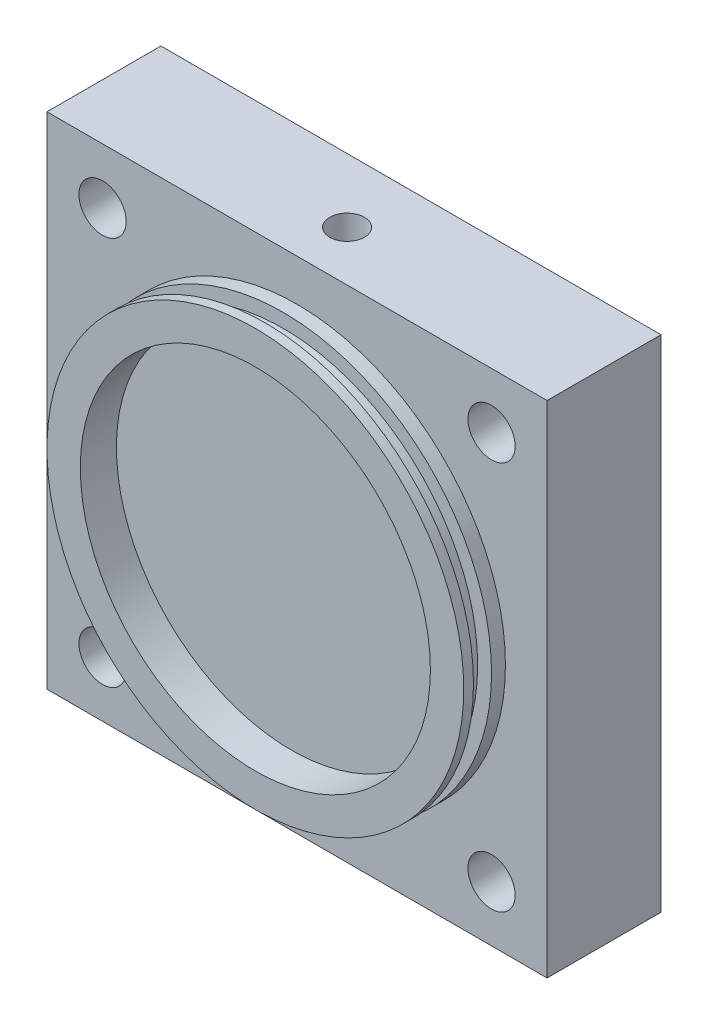
from build123d import *

# Parameters (mm, degrees)
SKETCH_1_W               = 180
SKETCH_1_H               = 180
EXTRUDE_1_DEPTH          = 41
SKETCH_2_R               = 75
EXTRUDE_2_DEPTH          = 15
SKETCH_3_R               = 63
CUT_EXTRUDE_1_DEPTH      = 13
SKETCH_4_W               = 6.5
SKETCH_4_H               = 5
CUT_EXTRUDE_2_REACH      = 136.347
CUT_EXTRUDE_2_END_RADIUS = 5.5626
SKETCH_9_R               = 3
CUT_EXTRUDE_4_REACH      = 141.054
SKETCH_11_R              = 8.5


with BuildPart() as part:
    # 草图1 → 凸台-拉伸1 (new body)
    with BuildSketch(Plane.XY):
        Rectangle(SKETCH_1_W, SKETCH_1_H)
    extrude(amount=EXTRUDE_1_DEPTH)

    # 草图2 → 凸台-拉伸2 (add)
    with BuildSketch(Plane.XY.offset(41)):
        Circle(SKETCH_2_R)
    extrude(amount=EXTRUDE_2_DEPTH)

    # 草图3 → 切除-拉伸1 (cut)
    with BuildSketch(Plane.XY.offset(56)):
        Circle(SKETCH_3_R)
    extrude(amount=-CUT_EXTRUDE_1_DEPTH, mode=Mode.SUBTRACT)

    # 草图4 → 切除-旋转1 (revolve, cut)
    with BuildSketch(Plane(origin=(0, 0, 0), x_dir=(0, 0, -1), z_dir=(1, 0, 0)), mode=Mode.PRIVATE) as cut_revolve_1_sk:
        with Locations((-49.25, 72.5)):
            Rectangle(SKETCH_4_W, SKETCH_4_H)
    revolve(cut_revolve_1_sk.sketch.rotate(Axis((0, 0, 56), (0, 0, -1)), 90), axis=Axis((0, 0, 56), (0, 0, -1)), mode=Mode.SUBTRACT)

    # 草图6 → 1/4 NPT 螺纹孔1 (revolve, cut)
    with BuildSketch(Plane(origin=(0, 90, 23), x_dir=(0, 0, 1), z_dir=(1, 0, 0))):
        Polygon((0, 0), (0, 36.342347279), (5.5626, 33), (5.5626, 10.02), (5.943676082, 10.02), (6.2436883, 0), align=None)
    revolve(axis=Axis((0, 96.35, 23), (0, -1, 0)), mode=Mode.SUBTRACT)

    # 切除-拉伸2: up to this cylinder (the profile starts outside it)
    cut_extrude_2_end = Plane(origin=(0, 60, 23), z_dir=(0, 1, 0)) * Cylinder(CUT_EXTRUDE_2_END_RADIUS, 284.8192, mode=Mode.PRIVATE)
    # 草图9 → 切除-拉伸2 (cut, up to the surface)
    with BuildSketch(Plane.XY.offset(43), mode=Mode.PRIVATE) as cut_extrude_2_sk1:
        with Locations(Location((0, 60, 0), (0, 0, 270))):
            Circle(SKETCH_9_R)
    cut_extrude_2_tool1 = extrude(cut_extrude_2_sk1.sketch, amount=-CUT_EXTRUDE_2_REACH, mode=Mode.PRIVATE) - cut_extrude_2_end
    add(cut_extrude_2_tool1.solids().sort_by_distance((0, 60, 43))[0], mode=Mode.SUBTRACT)

    # 草图11 → 切除-拉伸4 (cut, up to next)
    with BuildSketch(Plane(origin=(0, 0, 0), x_dir=(-1, 0, 0), z_dir=(0, 0, -1)), mode=Mode.PRIVATE) as cut_extrude_4_sk1:
        with Locations((-70, 70)):
            Circle(SKETCH_11_R)
    cut_extrude_4_tool1 = extrude(cut_extrude_4_sk1.sketch, amount=-CUT_EXTRUDE_4_REACH, mode=Mode.PRIVATE) & part.part
    # 草图11 → 切除-拉伸4 (cut, up to next)
    with BuildSketch(Plane(origin=(0, 0, 0), x_dir=(-1, 0, 0), z_dir=(0, 0, -1)), mode=Mode.PRIVATE) as cut_extrude_4_sk2:
        with Locations((70, 70)):
            Circle(SKETCH_11_R)
    cut_extrude_4_tool2 = extrude(cut_extrude_4_sk2.sketch, amount=-CUT_EXTRUDE_4_REACH, mode=Mode.PRIVATE) & part.part
    # 草图11 → 切除-拉伸4 (cut, up to next)
    with BuildSketch(Plane(origin=(0, 0, 0), x_dir=(-1, 0, 0), z_dir=(0, 0, -1)), mode=Mode.PRIVATE) as cut_extrude_4_sk3:
        with Locations((70, -70)):
            Circle(SKETCH_11_R)
    cut_extrude_4_tool3 = extrude(cut_extrude_4_sk3.sketch, amount=-CUT_EXTRUDE_4_REACH, mode=Mode.PRIVATE) & part.part
    # 草图11 → 切除-拉伸4 (cut, up to next)
    with BuildSketch(Plane(origin=(0, 0, 0), x_dir=(-1, 0, 0), z_dir=(0, 0, -1)), mode=Mode.PRIVATE) as cut_extrude_4_sk4:
        with Locations((-70, -70)):
            Circle(SKETCH_11_R)
    cut_extrude_4_tool4 = extrude(cut_extrude_4_sk4.sketch, amount=-CUT_EXTRUDE_4_REACH, mode=Mode.PRIVATE) & part.part
    add(cut_extrude_4_tool1.solids().sort_by_distance((70, 70, 0))[0], mode=Mode.SUBTRACT)
    add(cut_extrude_4_tool2.solids().sort_by_distance((-70, 70, 0))[0], mode=Mode.SUBTRACT)
    add(cut_extrude_4_tool3.solids().sort_by_distance((-70, -70, 0))[0], mode=Mode.SUBTRACT)
    add(cut_extrude_4_tool4.solids().sort_by_distance((70, -70, 0))[0], mode=Mode.SUBTRACT)


solid = part.part
